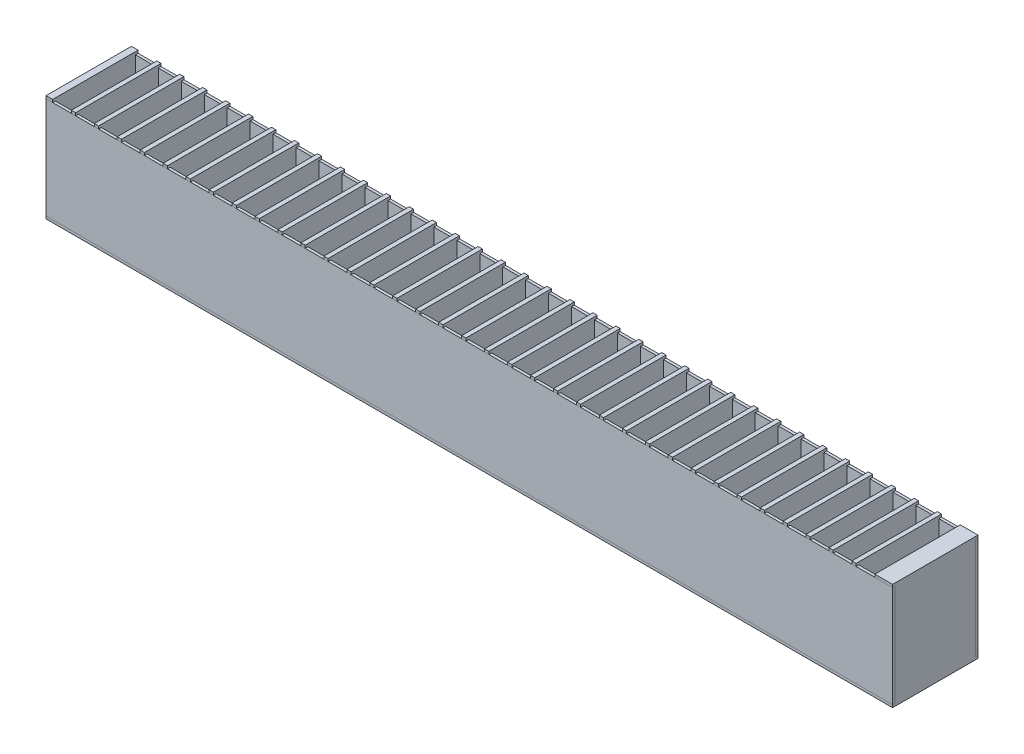
from build123d import *

# Parameters (mm, degrees)
SKETCH1_W             = 158.567646246
SKETCH1_H             = 16
SKETCH1_W_2           = 3.5
SKETCH1_H_2           = 5
BOSS_EXTRUDE1_DEPTH   = 10
CUT_EXTRUDE2_START    = -16
SKETCH4_W             = 3.5
SKETCH4_H             = 19.5
CUT_EXTRUDE2_DEPTH    = 16
CUT_EXTRUDE1_REACH    = 161.084
SKETCH2_W             = 0.5
SKETCH2_H             = 19
SKETCH3_W             = 0.5
SKETCH3_H             = 19
BOSS_EXTRUDE2_DEPTH   = 158.567646246
BOSS_EXTRUDE2_2_DEPTH = 158.567646246


with BuildPart() as part:
    # Sketch1 → Boss-Extrude1 (new, symmetric)
    with BuildSketch(Plane(origin=(0, 0, 0), x_dir=(1, 0, 0), z_dir=(0, 1, 0))):
        with Locations((1.039608447, 0)):
            Rectangle(SKETCH1_W, SKETCH1_H)
        with Locations((-2.15, -3.5)):
            Rectangle(SKETCH1_W_2, SKETCH1_H_2, mode=Mode.SUBTRACT)
        with Locations((-2.15, 3.5)):
            Rectangle(SKETCH1_W_2, SKETCH1_H_2, mode=Mode.SUBTRACT)
        with Locations((2.15, 3.5)):
            Rectangle(SKETCH1_W_2, SKETCH1_H_2, mode=Mode.SUBTRACT)
        with Locations((2.15, -3.5)):
            Rectangle(SKETCH1_W_2, SKETCH1_H_2, mode=Mode.SUBTRACT)
        with Locations((6.45, 3.5)):
            Rectangle(SKETCH1_W_2, SKETCH1_H_2, mode=Mode.SUBTRACT)
        with Locations((6.45, -3.5)):
            Rectangle(SKETCH1_W_2, SKETCH1_H_2, mode=Mode.SUBTRACT)
        with Locations((10.75, 3.5)):
            Rectangle(SKETCH1_W_2, SKETCH1_H_2, mode=Mode.SUBTRACT)
        with Locations((10.75, -3.5)):
            Rectangle(SKETCH1_W_2, SKETCH1_H_2, mode=Mode.SUBTRACT)
        with Locations((15.05, 3.5)):
            Rectangle(SKETCH1_W_2, SKETCH1_H_2, mode=Mode.SUBTRACT)
        with Locations((15.05, -3.5)):
            Rectangle(SKETCH1_W_2, SKETCH1_H_2, mode=Mode.SUBTRACT)
        with Locations((19.35, 3.5)):
            Rectangle(SKETCH1_W_2, SKETCH1_H_2, mode=Mode.SUBTRACT)
        with Locations((19.35, -3.5)):
            Rectangle(SKETCH1_W_2, SKETCH1_H_2, mode=Mode.SUBTRACT)
        with Locations((23.65, 3.5)):
            Rectangle(SKETCH1_W_2, SKETCH1_H_2, mode=Mode.SUBTRACT)
        with Locations((23.65, -3.5)):
            Rectangle(SKETCH1_W_2, SKETCH1_H_2, mode=Mode.SUBTRACT)
        with Locations((27.95, 3.5)):
            Rectangle(SKETCH1_W_2, SKETCH1_H_2, mode=Mode.SUBTRACT)
        with Locations((27.95, -3.5)):
            Rectangle(SKETCH1_W_2, SKETCH1_H_2, mode=Mode.SUBTRACT)
        with Locations((32.25, 3.5)):
            Rectangle(SKETCH1_W_2, SKETCH1_H_2, mode=Mode.SUBTRACT)
        with Locations((32.25, -3.5)):
            Rectangle(SKETCH1_W_2, SKETCH1_H_2, mode=Mode.SUBTRACT)
        with Locations((36.55, 3.5)):
            Rectangle(SKETCH1_W_2, SKETCH1_H_2, mode=Mode.SUBTRACT)
        with Locations((36.55, -3.5)):
            Rectangle(SKETCH1_W_2, SKETCH1_H_2, mode=Mode.SUBTRACT)
        with Locations((40.85, 3.5)):
            Rectangle(SKETCH1_W_2, SKETCH1_H_2, mode=Mode.SUBTRACT)
        with Locations((40.85, -3.5)):
            Rectangle(SKETCH1_W_2, SKETCH1_H_2, mode=Mode.SUBTRACT)
        with Locations((45.15, 3.5)):
            Rectangle(SKETCH1_W_2, SKETCH1_H_2, mode=Mode.SUBTRACT)
        with Locations((45.15, -3.5)):
            Rectangle(SKETCH1_W_2, SKETCH1_H_2, mode=Mode.SUBTRACT)
        with Locations((49.45, 3.5)):
            Rectangle(SKETCH1_W_2, SKETCH1_H_2, mode=Mode.SUBTRACT)
        with Locations((49.45, -3.5)):
            Rectangle(SKETCH1_W_2, SKETCH1_H_2, mode=Mode.SUBTRACT)
        with Locations((53.75, 3.5)):
            Rectangle(SKETCH1_W_2, SKETCH1_H_2, mode=Mode.SUBTRACT)
        with Locations((53.75, -3.5)):
            Rectangle(SKETCH1_W_2, SKETCH1_H_2, mode=Mode.SUBTRACT)
        with Locations((58.05, 3.5)):
            Rectangle(SKETCH1_W_2, SKETCH1_H_2, mode=Mode.SUBTRACT)
        with Locations((58.05, -3.5)):
            Rectangle(SKETCH1_W_2, SKETCH1_H_2, mode=Mode.SUBTRACT)
        with Locations((62.35, 3.5)):
            Rectangle(SKETCH1_W_2, SKETCH1_H_2, mode=Mode.SUBTRACT)
        with Locations((62.35, -3.5)):
            Rectangle(SKETCH1_W_2, SKETCH1_H_2, mode=Mode.SUBTRACT)
        with Locations((66.65, 3.5)):
            Rectangle(SKETCH1_W_2, SKETCH1_H_2, mode=Mode.SUBTRACT)
        with Locations((66.65, -3.5)):
            Rectangle(SKETCH1_W_2, SKETCH1_H_2, mode=Mode.SUBTRACT)
        with Locations((70.95, 3.5)):
            Rectangle(SKETCH1_W_2, SKETCH1_H_2, mode=Mode.SUBTRACT)
        with Locations((70.95, -3.5)):
            Rectangle(SKETCH1_W_2, SKETCH1_H_2, mode=Mode.SUBTRACT)
        with Locations((-6.45, 3.5)):
            Rectangle(SKETCH1_W_2, SKETCH1_H_2, mode=Mode.SUBTRACT)
        with Locations((-6.45, -3.5)):
            Rectangle(SKETCH1_W_2, SKETCH1_H_2, mode=Mode.SUBTRACT)
        with Locations((-10.75, 3.5)):
            Rectangle(SKETCH1_W_2, SKETCH1_H_2, mode=Mode.SUBTRACT)
        with Locations((-10.75, -3.5)):
            Rectangle(SKETCH1_W_2, SKETCH1_H_2, mode=Mode.SUBTRACT)
        with Locations((-15.05, 3.5)):
            Rectangle(SKETCH1_W_2, SKETCH1_H_2, mode=Mode.SUBTRACT)
        with Locations((-15.05, -3.5)):
            Rectangle(SKETCH1_W_2, SKETCH1_H_2, mode=Mode.SUBTRACT)
        with Locations((-19.35, 3.5)):
            Rectangle(SKETCH1_W_2, SKETCH1_H_2, mode=Mode.SUBTRACT)
        with Locations((-19.35, -3.5)):
            Rectangle(SKETCH1_W_2, SKETCH1_H_2, mode=Mode.SUBTRACT)
        with Locations((-23.65, 3.5)):
            Rectangle(SKETCH1_W_2, SKETCH1_H_2, mode=Mode.SUBTRACT)
        with Locations((-23.65, -3.5)):
            Rectangle(SKETCH1_W_2, SKETCH1_H_2, mode=Mode.SUBTRACT)
        with Locations((-27.95, 3.5)):
            Rectangle(SKETCH1_W_2, SKETCH1_H_2, mode=Mode.SUBTRACT)
        with Locations((-27.95, -3.5)):
            Rectangle(SKETCH1_W_2, SKETCH1_H_2, mode=Mode.SUBTRACT)
        with Locations((-32.25, 3.5)):
            Rectangle(SKETCH1_W_2, SKETCH1_H_2, mode=Mode.SUBTRACT)
        with Locations((-32.25, -3.5)):
            Rectangle(SKETCH1_W_2, SKETCH1_H_2, mode=Mode.SUBTRACT)
        with Locations((-36.55, 3.5)):
            Rectangle(SKETCH1_W_2, SKETCH1_H_2, mode=Mode.SUBTRACT)
        with Locations((-36.55, -3.5)):
            Rectangle(SKETCH1_W_2, SKETCH1_H_2, mode=Mode.SUBTRACT)
        with Locations((-40.85, 3.5)):
            Rectangle(SKETCH1_W_2, SKETCH1_H_2, mode=Mode.SUBTRACT)
        with Locations((-40.85, -3.5)):
            Rectangle(SKETCH1_W_2, SKETCH1_H_2, mode=Mode.SUBTRACT)
        with Locations((-45.15, 3.5)):
            Rectangle(SKETCH1_W_2, SKETCH1_H_2, mode=Mode.SUBTRACT)
        with Locations((-45.15, -3.5)):
            Rectangle(SKETCH1_W_2, SKETCH1_H_2, mode=Mode.SUBTRACT)
        with Locations((-49.45, 3.5)):
            Rectangle(SKETCH1_W_2, SKETCH1_H_2, mode=Mode.SUBTRACT)
        with Locations((-49.45, -3.5)):
            Rectangle(SKETCH1_W_2, SKETCH1_H_2, mode=Mode.SUBTRACT)
        with Locations((-53.75, 3.5)):
            Rectangle(SKETCH1_W_2, SKETCH1_H_2, mode=Mode.SUBTRACT)
        with Locations((-53.75, -3.5)):
            Rectangle(SKETCH1_W_2, SKETCH1_H_2, mode=Mode.SUBTRACT)
        with Locations((-58.05, 3.5)):
            Rectangle(SKETCH1_W_2, SKETCH1_H_2, mode=Mode.SUBTRACT)
        with Locations((-58.05, -3.5)):
            Rectangle(SKETCH1_W_2, SKETCH1_H_2, mode=Mode.SUBTRACT)
        with Locations((-62.35, 3.5)):
            Rectangle(SKETCH1_W_2, SKETCH1_H_2, mode=Mode.SUBTRACT)
        with Locations((-62.35, -3.5)):
            Rectangle(SKETCH1_W_2, SKETCH1_H_2, mode=Mode.SUBTRACT)
        with Locations((-66.65, 3.5)):
            Rectangle(SKETCH1_W_2, SKETCH1_H_2, mode=Mode.SUBTRACT)
        with Locations((-66.65, -3.5)):
            Rectangle(SKETCH1_W_2, SKETCH1_H_2, mode=Mode.SUBTRACT)
        with Locations((-70.95, 3.5)):
            Rectangle(SKETCH1_W_2, SKETCH1_H_2, mode=Mode.SUBTRACT)
        with Locations((-70.95, -3.5)):
            Rectangle(SKETCH1_W_2, SKETCH1_H_2, mode=Mode.SUBTRACT)
        with Locations((-75.25, 3.5)):
            Rectangle(SKETCH1_W_2, SKETCH1_H_2, mode=Mode.SUBTRACT)
        with Locations((-75.25, -3.5)):
            Rectangle(SKETCH1_W_2, SKETCH1_H_2, mode=Mode.SUBTRACT)
        with Locations((75.25, 3.5)):
            Rectangle(SKETCH1_W_2, SKETCH1_H_2, mode=Mode.SUBTRACT)
        with Locations((75.25, -3.5)):
            Rectangle(SKETCH1_W_2, SKETCH1_H_2, mode=Mode.SUBTRACT)
    extrude(amount=BOSS_EXTRUDE1_DEPTH, both=True)

    # Sketch4 → Cut-Extrude2 (cut)
    with BuildSketch(Plane.XY.offset(8).offset(CUT_EXTRUDE2_START)):
        with Locations((-2.15, 0.25)):
            Rectangle(SKETCH4_W, SKETCH4_H)
        with Locations((2.15, 0.25)):
            Rectangle(SKETCH4_W, SKETCH4_H)
        with Locations((6.45, 0.25)):
            Rectangle(SKETCH4_W, SKETCH4_H)
        with Locations((10.75, 0.25)):
            Rectangle(SKETCH4_W, SKETCH4_H)
        with Locations((15.05, 0.25)):
            Rectangle(SKETCH4_W, SKETCH4_H)
        with Locations((19.35, 0.25)):
            Rectangle(SKETCH4_W, SKETCH4_H)
        with Locations((23.65, 0.25)):
            Rectangle(SKETCH4_W, SKETCH4_H)
        with Locations((27.95, 0.25)):
            Rectangle(SKETCH4_W, SKETCH4_H)
        with Locations((32.25, 0.25)):
            Rectangle(SKETCH4_W, SKETCH4_H)
        with Locations((36.55, 0.25)):
            Rectangle(SKETCH4_W, SKETCH4_H)
        with Locations((40.85, 0.25)):
            Rectangle(SKETCH4_W, SKETCH4_H)
        with Locations((45.15, 0.25)):
            Rectangle(SKETCH4_W, SKETCH4_H)
        with Locations((49.45, 0.25)):
            Rectangle(SKETCH4_W, SKETCH4_H)
        with Locations((53.75, 0.25)):
            Rectangle(SKETCH4_W, SKETCH4_H)
        with Locations((58.05, 0.25)):
            Rectangle(SKETCH4_W, SKETCH4_H)
        with Locations((62.35, 0.25)):
            Rectangle(SKETCH4_W, SKETCH4_H)
        with Locations((66.65, 0.25)):
            Rectangle(SKETCH4_W, SKETCH4_H)
        with Locations((70.95, 0.25)):
            Rectangle(SKETCH4_W, SKETCH4_H)
        with Locations((75.25, 0.25)):
            Rectangle(SKETCH4_W, SKETCH4_H)
        with Locations((-6.45, 0.25)):
            Rectangle(SKETCH4_W, SKETCH4_H)
        with Locations((-10.75, 0.25)):
            Rectangle(SKETCH4_W, SKETCH4_H)
        with Locations((-15.05, 0.25)):
            Rectangle(SKETCH4_W, SKETCH4_H)
        with Locations((-19.35, 0.25)):
            Rectangle(SKETCH4_W, SKETCH4_H)
        with Locations((-23.65, 0.25)):
            Rectangle(SKETCH4_W, SKETCH4_H)
        with Locations((-27.95, 0.25)):
            Rectangle(SKETCH4_W, SKETCH4_H)
        with Locations((-32.25, 0.25)):
            Rectangle(SKETCH4_W, SKETCH4_H)
        with Locations((-36.55, 0.25)):
            Rectangle(SKETCH4_W, SKETCH4_H)
        with Locations((-40.85, 0.25)):
            Rectangle(SKETCH4_W, SKETCH4_H)
        with Locations((-45.15, 0.25)):
            Rectangle(SKETCH4_W, SKETCH4_H)
        with Locations((-49.45, 0.25)):
            Rectangle(SKETCH4_W, SKETCH4_H)
        with Locations((-53.75, 0.25)):
            Rectangle(SKETCH4_W, SKETCH4_H)
        with Locations((-58.05, 0.25)):
            Rectangle(SKETCH4_W, SKETCH4_H)
        with Locations((-62.35, 0.25)):
            Rectangle(SKETCH4_W, SKETCH4_H)
        with Locations((-66.65, 0.25)):
            Rectangle(SKETCH4_W, SKETCH4_H)
        with Locations((-70.95, 0.25)):
            Rectangle(SKETCH4_W, SKETCH4_H)
        with Locations((-75.25, 0.25)):
            Rectangle(SKETCH4_W, SKETCH4_H)
    cut_extrude2 = extrude(amount=CUT_EXTRUDE2_DEPTH, mode=Mode.SUBTRACT)

    # Mirror1: Cut-Extrude2 across plane
    add(cut_extrude2.mirror(Plane.XY), mode=Mode.SUBTRACT)

    # Cut-Extrude1: up to this face of the body (flat: up to its plane)
    cut_extrude1_end = Plane(part.part.faces().sort_by_distance((-78.244214676, 0, 0))[0])
    # Sketch2 → Cut-Extrude1 (cut, up to the picked face)
    with BuildSketch(Plane(origin=(80.32343157, 0, 0), x_dir=(0, 0, -1), z_dir=(1, 0, 0)), mode=Mode.PRIVATE) as cut_extrude1_sk1:
        with Locations((-7.75, 0)):
            Rectangle(SKETCH2_W, SKETCH2_H)
    cut_extrude1_tool1 = split(extrude(cut_extrude1_sk1.sketch, amount=-CUT_EXTRUDE1_REACH, mode=Mode.PRIVATE), bisect_by=cut_extrude1_end, keep=Keep.BOTH, mode=Mode.PRIVATE)
    # Sketch2 → Cut-Extrude1 (cut, up to the picked face)
    with BuildSketch(Plane(origin=(80.32343157, 0, 0), x_dir=(0, 0, -1), z_dir=(1, 0, 0)), mode=Mode.PRIVATE) as cut_extrude1_sk2:
        with Locations((7.75, 0)):
            Rectangle(SKETCH2_W, SKETCH2_H)
    cut_extrude1_tool2 = split(extrude(cut_extrude1_sk2.sketch, amount=-CUT_EXTRUDE1_REACH, mode=Mode.PRIVATE), bisect_by=cut_extrude1_end, keep=Keep.BOTH, mode=Mode.PRIVATE)
    add(cut_extrude1_tool1.solids().sort_by(Axis((80.323432, 0, 7.75), (-1, 0, 0)))[0], mode=Mode.SUBTRACT)
    add(cut_extrude1_tool2.solids().sort_by(Axis((80.323432, 0, -7.75), (-1, 0, 0)))[0], mode=Mode.SUBTRACT)


with BuildPart() as body_2:
    # Sketch3 → Boss-Extrude2 (new body)
    with BuildSketch(Plane(origin=(80.32343157, 0, 0), x_dir=(0, 0, -1), z_dir=(1, 0, 0))):
        with Locations((-7.75, 0)):
            Rectangle(SKETCH3_W, SKETCH3_H)
    extrude(amount=-BOSS_EXTRUDE2_DEPTH)


with BuildPart() as body_3:
    # Sketch3 → Boss-Extrude2 2 (new body)
    with BuildSketch(Plane(origin=(80.32343157, 0, 0), x_dir=(0, 0, -1), z_dir=(1, 0, 0))):
        with Locations((7.75, 0)):
            Rectangle(SKETCH3_W, SKETCH3_H)
    extrude(amount=-BOSS_EXTRUDE2_2_DEPTH)


solid = Compound([part.part, body_2.part, body_3.part])
